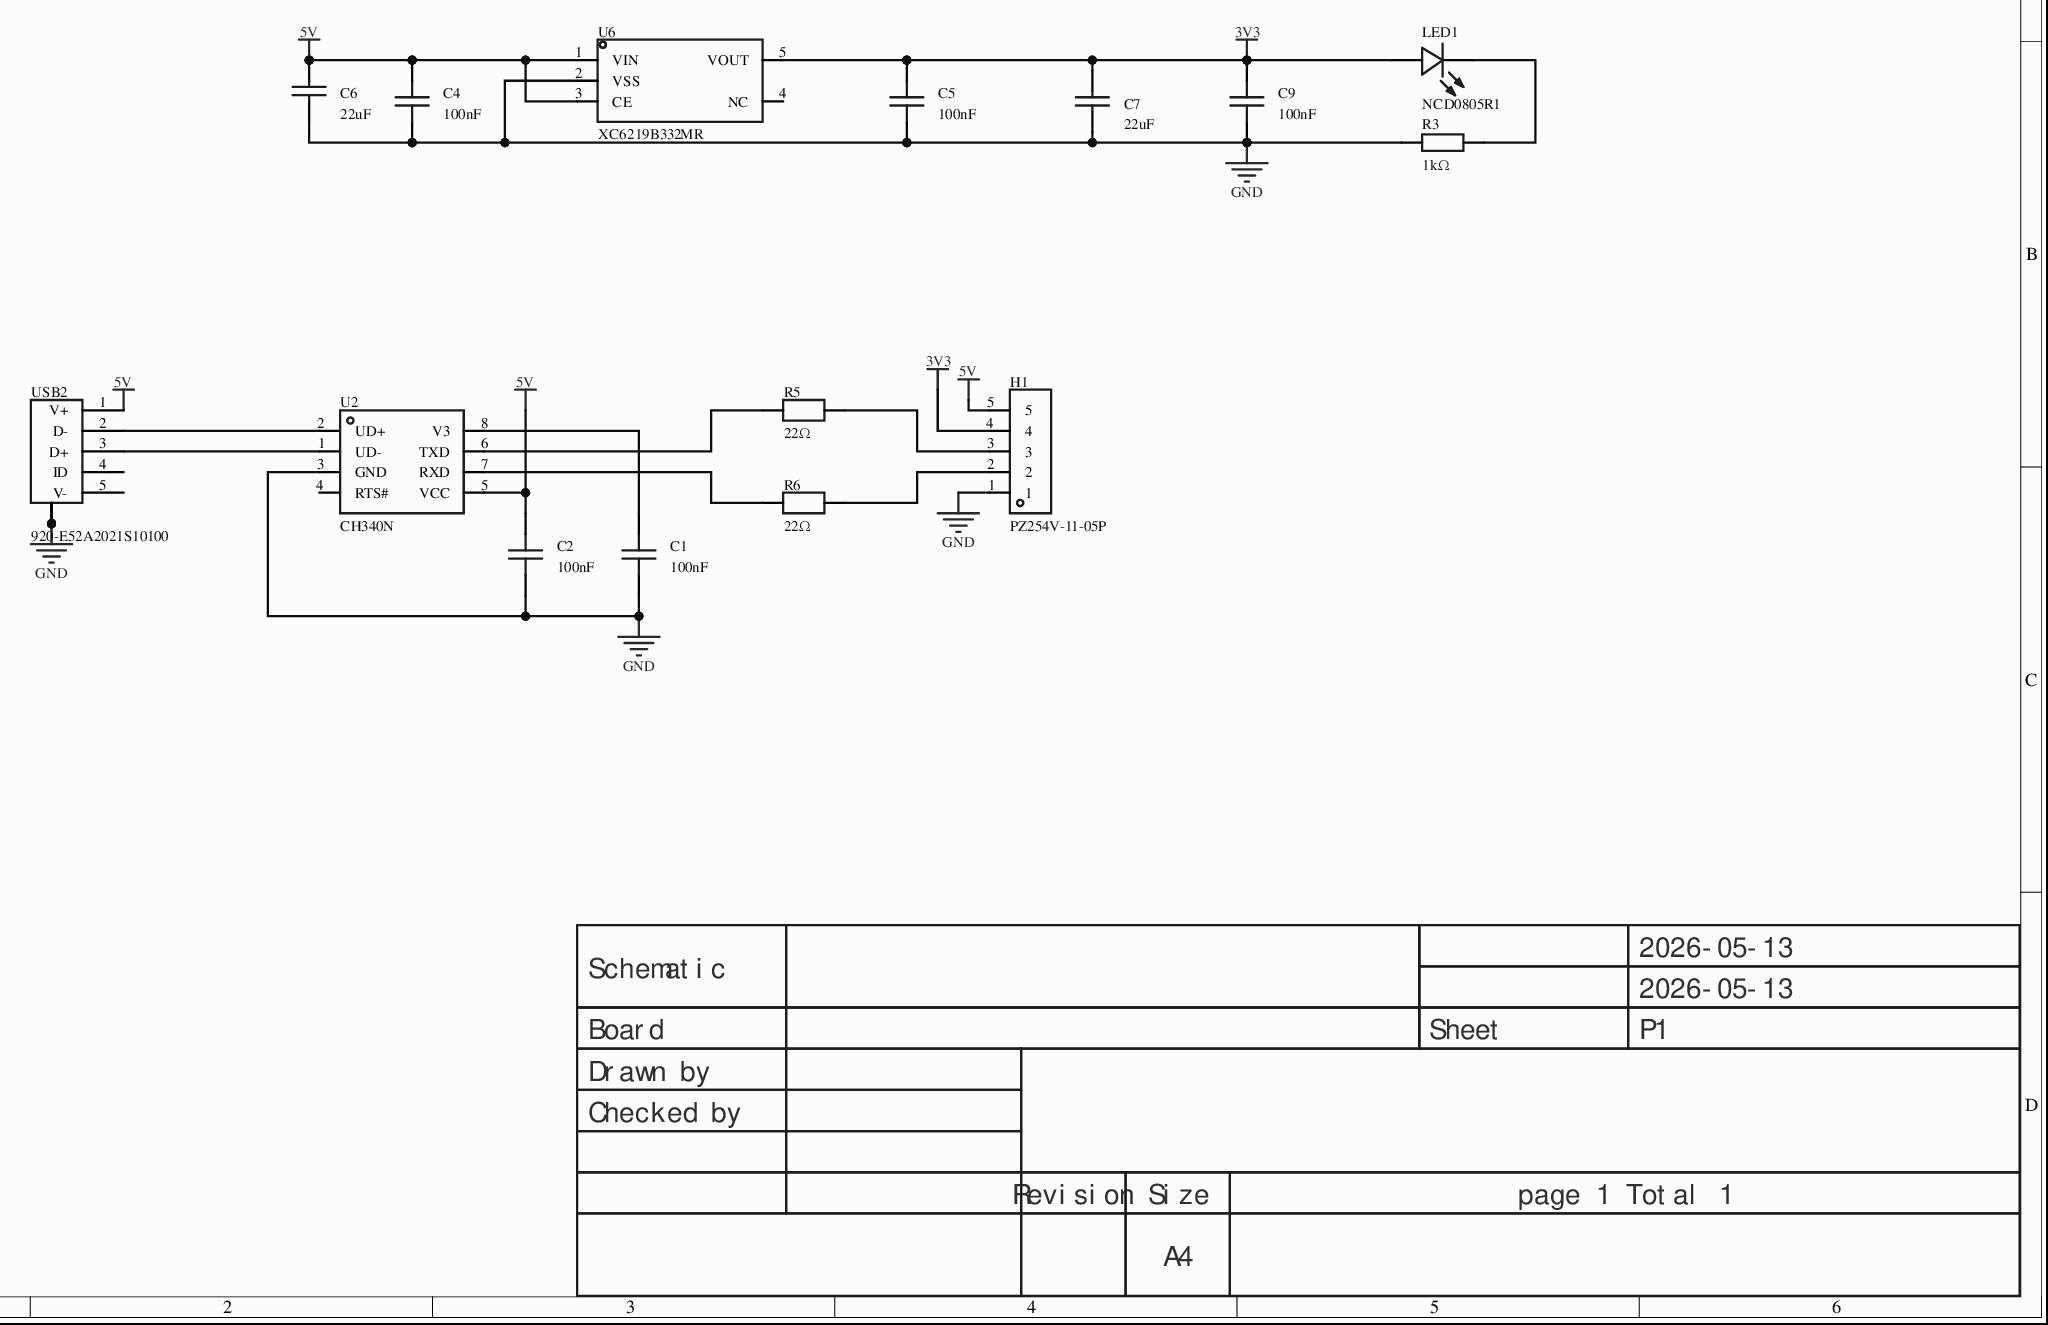
[diagram p0: MISC89035-3.schdoc]
# Altium project MISC89035-2.PrjPcb
1 sheet, 15 parts. Net scope: global (net labels, ports and power ports of the same name join across sheets).
Board file: MISC89035.pcbdoc

## Sheet MISC89035-3.schdoc
size 297 x 209 mm; Version: V1.0; @Project Name: MISC89035; @Update Date: 2026-05-13; @Create Date: 2026-05-13; @Board Name: MISC89035; @Create Time: 09:10:08; @Page Count: 1; @Page No: 1; @Schematic Name: MISC89035; @Update Time: 09:10:08; Size: A4

### Parts
C1  100nF  [C0603]
C2  100nF  [C0603]
C4  100nF  [C0603]
C5  100nF  [C0603]
C6  22uF  [C0805]
C7  22uF  [C0805]
C9  100nF  [C0603]
H1  PZ254V-11-05P  [HDR-TH_5P-P2.54-V-M]
LED1  NCD0805R1  [LED0805-RD]
R3  1kΩ  [R0603]
R5  22Ω  [R0603]
R6  22Ω  [R0603]
U2  CH340N  [SOP-8_L4.9-W3.9-P1.27-LS6.0-BL]
U6  XC6219B332MR  [SOT-23-5_L3.0-W1.7-P0.95-LS2.8-BR]
USB2  920-E52A2021S10100  [MICRO-USB-SMD_5P-P0.65-H-F_C10418]

### Nets
3V3: C5.2 C7.2 C9.2 H1.4 LED1.2(+) U6.5(VOUT)
5V: C2.2 C4.2 C6.2 H1.5 U2.5(VCC) U6.1(VIN) U6.3(CE) USB2.1(V+)
GND: C1.1 C2.1 C4.1 C5.1 C6.1 C7.1 C9.1 H1.1 R3.1 U2.3(GND) U6.2(VSS) USB2.SH0(MTN) USB2.SH1 USB2.SH2 USB2.SH3
NetC1_2: C1.2 U2.8(V3)
NetH1_2: H1.2 R6.2
NetH1_3: H1.3 R5.2
NetLED1_1: LED1.1(-) R3.2
NetR5_1: R5.1 U2.6(TXD)
NetR6_1: R6.1 U2.7(RXD)
NetU2_1: U2.1(UD-) USB2.3(D+)
NetU2_2: U2.2(UD+) USB2.2(D-)

Not connected (* = marked no-connect by the designer): U2 4(RTS#); U6 4(NC); USB2 4(ID) 5(V-)

### Notes on the sheet
- 2026-05-13
- Schematic
- Board
- Sheet
- P1
- Drawn by
- Checked by
- Revision
- Size
- A4
- page 1 Total 1

### Library data of the parts
C1 C2 C4 C9 = CC0603KRX7R9BB104: Capacitance:100nF;Tolerance:±10%;Rated voltage:50V;Temperature coefficient:X7R;; Manufacturer: YAGEO(国巨); AddInBom: yes; ModelId: ac125912035d415993ca9572d50418b10819f05c4eef4c71ace90d822a990e87; ModelName: C0603_L1.6-W0.8-H0.8; ModelTransform: 62.992,31.496,0,0,0,0,0,0,0; Tolerance: ±10%; Voltage Rating: 50V; Temperature Coefficient: X7R; Symbol: CC0603KRX7R9BB104; Device: CC0603KRX7R9BB104; LCSC Part Name: 100nF ±10% 50V; SupplierPart: C14663; ManufacturerPart: CC0603KRX7R9BB104; Supplier Footprint: 0603; JLCPCB Part Class: Basic Part; Datasheet: https://example.com/datasheet/CC0603KRX7R9BB104/15331.html; Supplier: LCSC; ConvertToPcb: yes; FootprintName: C0603; Value: 100nF
C5 = 0603BB104K500NGT: Capacitance:100nF;Tolerance:±10%;Rated voltage:50V;Temperature coefficient (material):X7R;; Manufacturer: Knowles(楼氏); AddInBom: yes; ModelId: ac125912035d415993ca9572d50418b10819f05c4eef4c71ace90d822a990e87; ModelName: C0603_L1.6-W0.8-H0.8; ModelTransform: 62.992,31.496,0,0,0,0,0,0,0; Tolerance: ±10%; Voltage Rated: 50V; Temperature Coefficient: X7R; Symbol: 0603BB104K500NGT; Device: 0603BB104K500NGT; LCSC Part Name: 100nF ±10% 50V; SupplierPart: C2168571; ManufacturerPart: 0603BB104K500NGT; Supplier Footprint: 0603; JLCPCB Part Class: Extended Part; Datasheet: https://example.com/upload/public/pdf/source/20210426/55B82DB4A9EC19DEFEE13887341FCC08.pdf; Supplier: LCSC; ConvertToPcb: yes; FootprintName: C0603; Value: 100nF
C6 C7 = 0805X226M6R3NT: Capacitance:22uF;Tolerance:±20%;Rated voltage:6.3V;Temperature coefficient:X5R;; Manufacturer: FH(风华); AddInBom: yes; ModelId: 1ba041120af144c991958decab20d2410819f05c4eef4c71ace90d822a990e87; ModelName: C0805_L2.0-W1.3-H1.3; ModelTransform: 78.74,51.181,0,0,0,0,0,0.0005,0; Tolerance: ±20%; Voltage Rating: 6.3V; Temperature Coefficient: X5R; Symbol: 0805X226M6R3NT; Device: 0805X226M6R3NT; LCSC Part Name: 22uF ±20% 6.3V; SupplierPart: C105484; ManufacturerPart: 0805X226M6R3NT; Supplier Footprint: 0805; JLCPCB Part Class: Extended Part; Datasheet: https://example.com/datasheet/0805X226M6R3NT/106699.html; Supplier: LCSC; ConvertToPcb: yes; FootprintName: C0805; Value: 22uF
H1 = PZ254V-11-05P: Pin structure:1x5P;Pitch:2.54mm;Row spacing:-;Square/round pin:Square pin;Mounting:Through-hole;Rows:Single row;Total pins:5P;Rated current:3A;Rated voltage:250V;Mating pin length:6mm;Plastic height:2.5mm;Termination pin length:3mm;Contact material:Brass;Contact plating:-;Operating temperature:-40℃~+105℃;Color:Black;; Manufacturer: XFCN(兴飞); AddInBom: yes; ModelId: 47d466e4a34f4fc5bc626cf773a24dd50819f05c4eef4c71ace90d822a990e87; ModelName: HDR-TH_5P-P2.54-M-LI-1X5P; ModelTransform: 499.999,100,0,0,0,0,0,0,-118.11; Pin Structure: 1x5P; Pitch: 2.54mm; Current Rating: 3A; Voltage Rating (Max): 250V; Symbol: PZ254V-11-05P; Device: PZ254V-11-05P; LCSC Part Name: 1x5P 间距:2.54mm 方针 直插; SupplierPart: C492404; ManufacturerPart: PZ254V-11-05P; Supplier Footprint: 插件,P=2.54mm; JLCPCB Part Class: Extended Part; Datasheet: https://example.com/datasheet/PZ254V-11-05P/502960.html; Supplier: LCSC; ConvertToPcb: yes; FootprintName: HDR-TH_5P-P2.54-V-M; Row Spacing: -; Circluar Pins/Square Pins: Square pin; Mounting Type: Through-hole; Number of Rows: Single row; Number of Pins: 5P; Length of Mating Pin: 6mm; Insulation Height: 2.5mm; Length of End Connection Pin: 3mm; Contact Material: Brass; Contact Plating: -; Operating Temperature: -40℃~+105℃; Color: Black
LED1 = NCD0805R1: Lamp head type:-;Emitted color:Red;Forward voltage (Vf):1.6V~2.6V;Power:65mW;Forward current:25mA;Wavelength:615nm~630nm;Diode configuration:Single diode;Lens color:-;Color temperature:-;Luminous intensity:195mcd;Viewing angle:130°;Tape packaging:-;Operating temperature:-30℃~+85℃;; Manufacturer: 国星光电; Symbol: FC-2012HRK-620D; AddInBom: yes; ModelId: b1c5ed7a4f6e46d3bc6f6cc7c20f3fea0819f05c4eef4c71ace90d822a990e87; ModelTransform: 79.527,49.2125,0,0,0,0,0,0,0; Illumination Color: Red; Power(Watts): 65mW; Forward Current: 25mA; Peak Wavelength: 630nm; Luminous Intensity: 195mcd; Viewing Angle: 130°; Device: NCD0805R1; LCSC Part Name: 片式发光二极管; SupplierPart: C84256; ManufacturerPart: NCD0805R1; Supplier Footprint: 0805; JLCPCB Part Class: Basic Part; Datasheet: https://example.com/datasheet/NCD0805R1/85425.html; Supplier: LCSC; ConvertToPcb: yes; FootprintName: LED0805-RD; ModelName: LED0805-RD; Lamp Holder Type: -; Voltage - Forward(Vf): 1.6V~2.6V; Wavelength - Dominant: 615nm~630nm; Diode Configuration: Single diode; Lens Color: -; Color Temperature: -; Mounting Style: -; Operating Temperature: -30℃~+85℃
R3 = 0603WAF1001T5E: Resistor type:Thick film resistor;Resistance:1kΩ;Tolerance:±1%;Power:100mW;Operating voltage:75V;Temperature coefficient:±100ppm/℃;; Manufacturer: UNI-ROYAL(厚声); AddInBom: yes; ModelId: fc143cca1e79419f9cd78b61e9279f080819f05c4eef4c71ace90d822a990e87; ModelTransform: 31.8897,63.7794,0,90,0,0,0,0,0; Tolerance: ±1%; Power(Watts): 100mW; Voltage-Supply(Max): 75V; Symbol: 0603WAF1001T5E; Device: 0603WAF1001T5E; LCSC Part Name: 1kΩ ±1% 100mW 厚膜电阻; SupplierPart: C21190; ManufacturerPart: 0603WAF1001T5E; Supplier Footprint: 0603; JLCPCB Part Class: Basic Part; Datasheet: https://example.com/datasheet/0603WAF1001T5E/21904.html; Supplier: LCSC; ConvertToPcb: yes; FootprintName: R0603; ModelName: R0603; Type: Thick film resistor; Value: 1kΩ; Temperature Coefficient: ±100ppm/℃; Operating Temperature: -55℃~+155℃
R5 R6 = SCR0603J22R: Resistor type:Thick film resistor;Resistance:22Ω;Tolerance:±5%;Power:100mW;Maximum operating voltage:75V;; Manufacturer: VO(翔胜); AddInBom: yes; ModelId: fc143cca1e79419f9cd78b61e9279f080819f05c4eef4c71ace90d822a990e87; ModelTransform: 31.8897,63.7794,0,90,0,0,0,0,0; Tolerance: ±5%; Power(Watts): 100mW; Overload Voltage (Max): 75V; Symbol: SCR0603J22R; Device: SCR0603J22R; LCSC Part Name: 厚膜电阻 22Ω ±5% 100mW; SupplierPart: C3017773; ManufacturerPart: SCR0603J22R; Supplier Footprint: 0603; JLCPCB Part Class: Extended Part; Datasheet: https://example.com/upload/public/pdf/source/20220513/247AF9639BA21CF93567DC289CCC6A22.pdf; Supplier: LCSC; ConvertToPcb: yes; FootprintName: R0603; ModelName: R0603; Type: Thick film resistor; Value: 22Ω; Operating Temperature Range: -55℃~+155℃
U2 = CH340N: Application function:USB to serial;USB protocol version:USB 2.0;Channels:1;Data rate:2Mbps;; Manufacturer: WCH(南京沁恒); Symbol: CH340N_C2977777_2; AddInBom: yes; ModelId: 75c24a7891ee4dd6bdac16a7163ff87e0819f05c4eef4c71ace90d822a990e87; ModelName: SOP-8_L4.9-W3.9-P1.27-LS6.0-BL-1; ModelTransform: 192.913,236.22,0,0,0,0,-0.393,2.749,0; USB Protocol: USB 2.0; Number of Channels: 1; Voltage - Supply: 3.3V; 5V; Data Rate: 2Mbps; Device: CH340N; LCSC Part Name: USB2.0芯片CH340; SupplierPart: C2977777; ManufacturerPart: CH340N; Supplier Footprint: SOP-8; JLCPCB Part Class: Extended Part; Datasheet: https://example.com/datasheet/CH340N/3390257.html; Supplier: LCSC; ConvertToPcb: yes; FootprintName: SOP-8_L4.9-W3.9-P1.27-LS6.0-BL; Applications Function: USB to serial; Operating Temperature: -20℃~+70℃
U6 = XC6219B332MR_C347386: Output type:Fixed;Operating voltage:7V;Output voltage:3.3V;Output current:300mA;Power supply rejection ratio (PSRR):40dB@(1kHz);Output polarity:Positive;; Manufacturer: UMW(友台半导体); AddInBom: yes; ModelId: 0a2a1b8f50944f73965918ad6e5fe1670819f05c4eef4c71ace90d822a990e87; ModelName: SOT-23-5_L2.9-W1.6-H1.1-LS2.8-P0.95; ModelTransform: 114.173,109.636,0,180,0,0,0,0,0; Output Type: Fixed; Voltage - Supply: 7V; Output Voltage: 3.3V; Output Current: 300mA; Voltage Dropout: 280mV@(100mA); standby current: 15uA; Number of Outputs: 1; Symbol: XC6219B332MR_C347386; Device: XC6219B332MR_C347386; LCSC Part Name: 输入7V 输出3.3V 300mA; SupplierPart: C347386; ManufacturerPart: XC6219B332MR; Supplier Footprint: SOT-23-5; JLCPCB Part Class: Extended Part; Datasheet: https://example.com/datasheet/XC6219B332MR/324046.html; Supplier: LCSC; ConvertToPcb: yes; FootprintName: SOT-23-5_L3.0-W1.7-P0.95-LS2.8-BR; Power Supply Rejection Ratio (PSRR): 40dB@(1kHz); Features: Overcurrent protection; enable; short-circuit protection; Operating Temperature: -20℃~+60℃; Output Configuration: Positive
USB2 = 920-E52A2021S10100: Connector type:Micro-B;Protocol standard:USB 2.0;Gender:Female;Mounting:Horizontal mount;Contact count:5P;Port count:1;Rated current - power:1A;Operating temperature:-30℃~+80℃;; Manufacturer: 精拓金; Symbol: micro USBFemale; AddInBom: yes; ModelId: 8d98bdb22dfe41cea8df3303517703a80819f05c4eef4c71ace90d822a990e87; ModelTransform: 315.054,220.472,0,180,0,0,0,-51.038,-39.37; Protocol Standard: USB 2.0; Gender: Female; Number of Contacts: 5P; Number of Ports: 1; Current Rating-Power: 1A; Detection color: Black; Device: 920-E52A2021S10100; LCSC Part Name: Micro-B 母 卧贴; SupplierPart: C10418; ManufacturerPart: 920-E52A2021S10100; Supplier Footprint: SMD; JLCPCB Part Class: Extended Part; Datasheet: https://example.com/datasheet/920-E52A2021S10100/10961.html; Supplier: LCSC; ConvertToPcb: yes; FootprintName: MICRO-USB-SMD_5P-P0.65-H-F_C10418; ModelName: MICRO-USB-SMD_5P-P0.65-H-F_C10418; Connector Type: Micro-B; Mounting Type: Horizontal mount; Length: 5.15mm; Operating Temperature: -30℃~+80℃